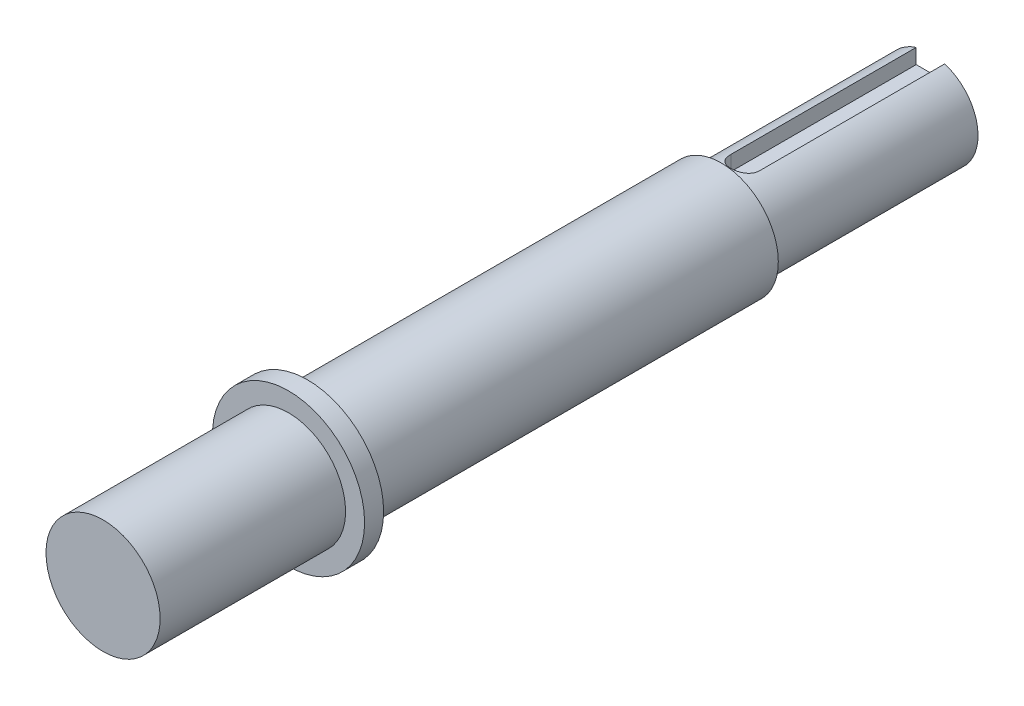
SolidWorks part; units mm, degrees
ref_plane "前视基准面" through (0, 0, 0) normal (0, 0, 1) x (1, 0, 0)
ref_plane "上视基准面" through (0, 0, 0) normal (0, 1, 0) x (1, 0, 0)
ref_plane "右视基准面" through (0, 0, 0) normal (1, 0, 0) x (0, 0, -1)
sketch "草图1" plane through (0, 0, 0) normal (0, 0, 1) x (1, 0, 0)
  circle A0 centre (0, 0) radius 6
  dimension "D1" = 12
extrude "凸台-拉伸1" add sketch "草图1" along normal blind 65
cosmetic thread "装饰螺纹线1" parameters "D1"=15, "D2"=10.106
sketch "草图2" plane through (0, 0, 0) normal (0, 0, -1) x (-1, 0, 0)
  circle A0 centre (0, 0) radius 5
  dimension "D1" = 10
extrude "凸台-拉伸2" add sketch "草图2" along normal blind 22
sketch "草图3" plane through (0, 0, 0) normal (0, 1, 0) x (1, 0, 0)
  line L0 (-6, 0) -> (-6, -65) construction
  line L1 (-6, -43.5) -> (-8, -43.5)
  line L2 (-6, -43.5) -> (-6, -45.5)
  line L3 (-6, -45.5) -> (-8, -45.5)
  line L4 (-8, -43.5) -> (-8, -45.5)
  line L5 (-6, -65) -> (6, -65) construction
  line L6 (0, -65) -> (0, -17.4586) construction
  dimension "D1" = 21.5
  dimension "D2" = 2
  dimension "D3" = 2
revolve "旋转1" add sketch "草图3" angle 360 about L6
sketch "MyToolsJD" plane through (0, 0, -22) normal (0, 0, -1) x (-1, 0, 0)
  line L0 (0, 0) -> (5, 0) construction
  line L1 (0, 0) -> (0, 5) construction
  circle A0 centre (0, 0) radius 5 construction
  circle A1 centre (0, 0) radius 5 construction
  dimension "D1" = 90
ref_plane "基准面1" through (0, 5, -22) normal (0, 1, 0) x (0, 0, 1)
sketch "MyToolsZJC" plane through (0, 5, -22) normal (0, 1, 0) x (0, 0, 1)
  line L0 (-0.5, 0) -> (19.5, 0) construction
  line L1 (-0.5, 1.5) -> (19.5, 1.5)
  line L2 (-0.5, -1.5) -> (19.5, -1.5)
  line L3 (0, 0) -> (-0.5, 0) construction
  arc A0 (-0.5, 1.5) -> (-0.5, -1.5) centre (-0.5, 0) ccw
  arc A1 (19.5, -1.5) -> (19.5, 1.5) centre (19.5, 0) ccw
  point P2 (9.5, 0)
  point P13 (21, 0)
  point P14 (-2, 0)
  dimension "D3" = 23
  dimension "D1" = 3
  dimension "D2" = 0.5
extrude "ZJCQC" cut sketch "MyToolsZJC" against normal blind 1.8
sketch "草图10" plane through (0, 0, -22) normal (0, 0, -1) x (-1, 0, 0)
  point P0 (0, 0)
hole_wizard "M4 螺纹孔1" positions "草图10" profile "草图9" tap size "M4" standard "GB"
sketch "草图9" plane through (0, 0, -22) normal (1, 0, 0) x (0, 1, 0)
  line L0 (0, 0) -> (0, 11.0914)
  line L1 (0, 11.0914) -> (1.65, 10.1)
  line L2 (1.65, 10.1) -> (1.65, 0)
  line L5 (1.65, 0) -> (0, 0)
  line L10 (0, 11.0914) -> (-1.65, 10.1) construction
  line L11 (0, -6.35) -> (0, 107.95) construction
  dimension "螺纹孔钻头直径" = 3.3
  dimension "螺纹孔钻头深度" = 10.1
  dimension "导头角度" = 118
cosmetic thread "孔螺纹线1" parameters "D1"=8, "D2"=4
